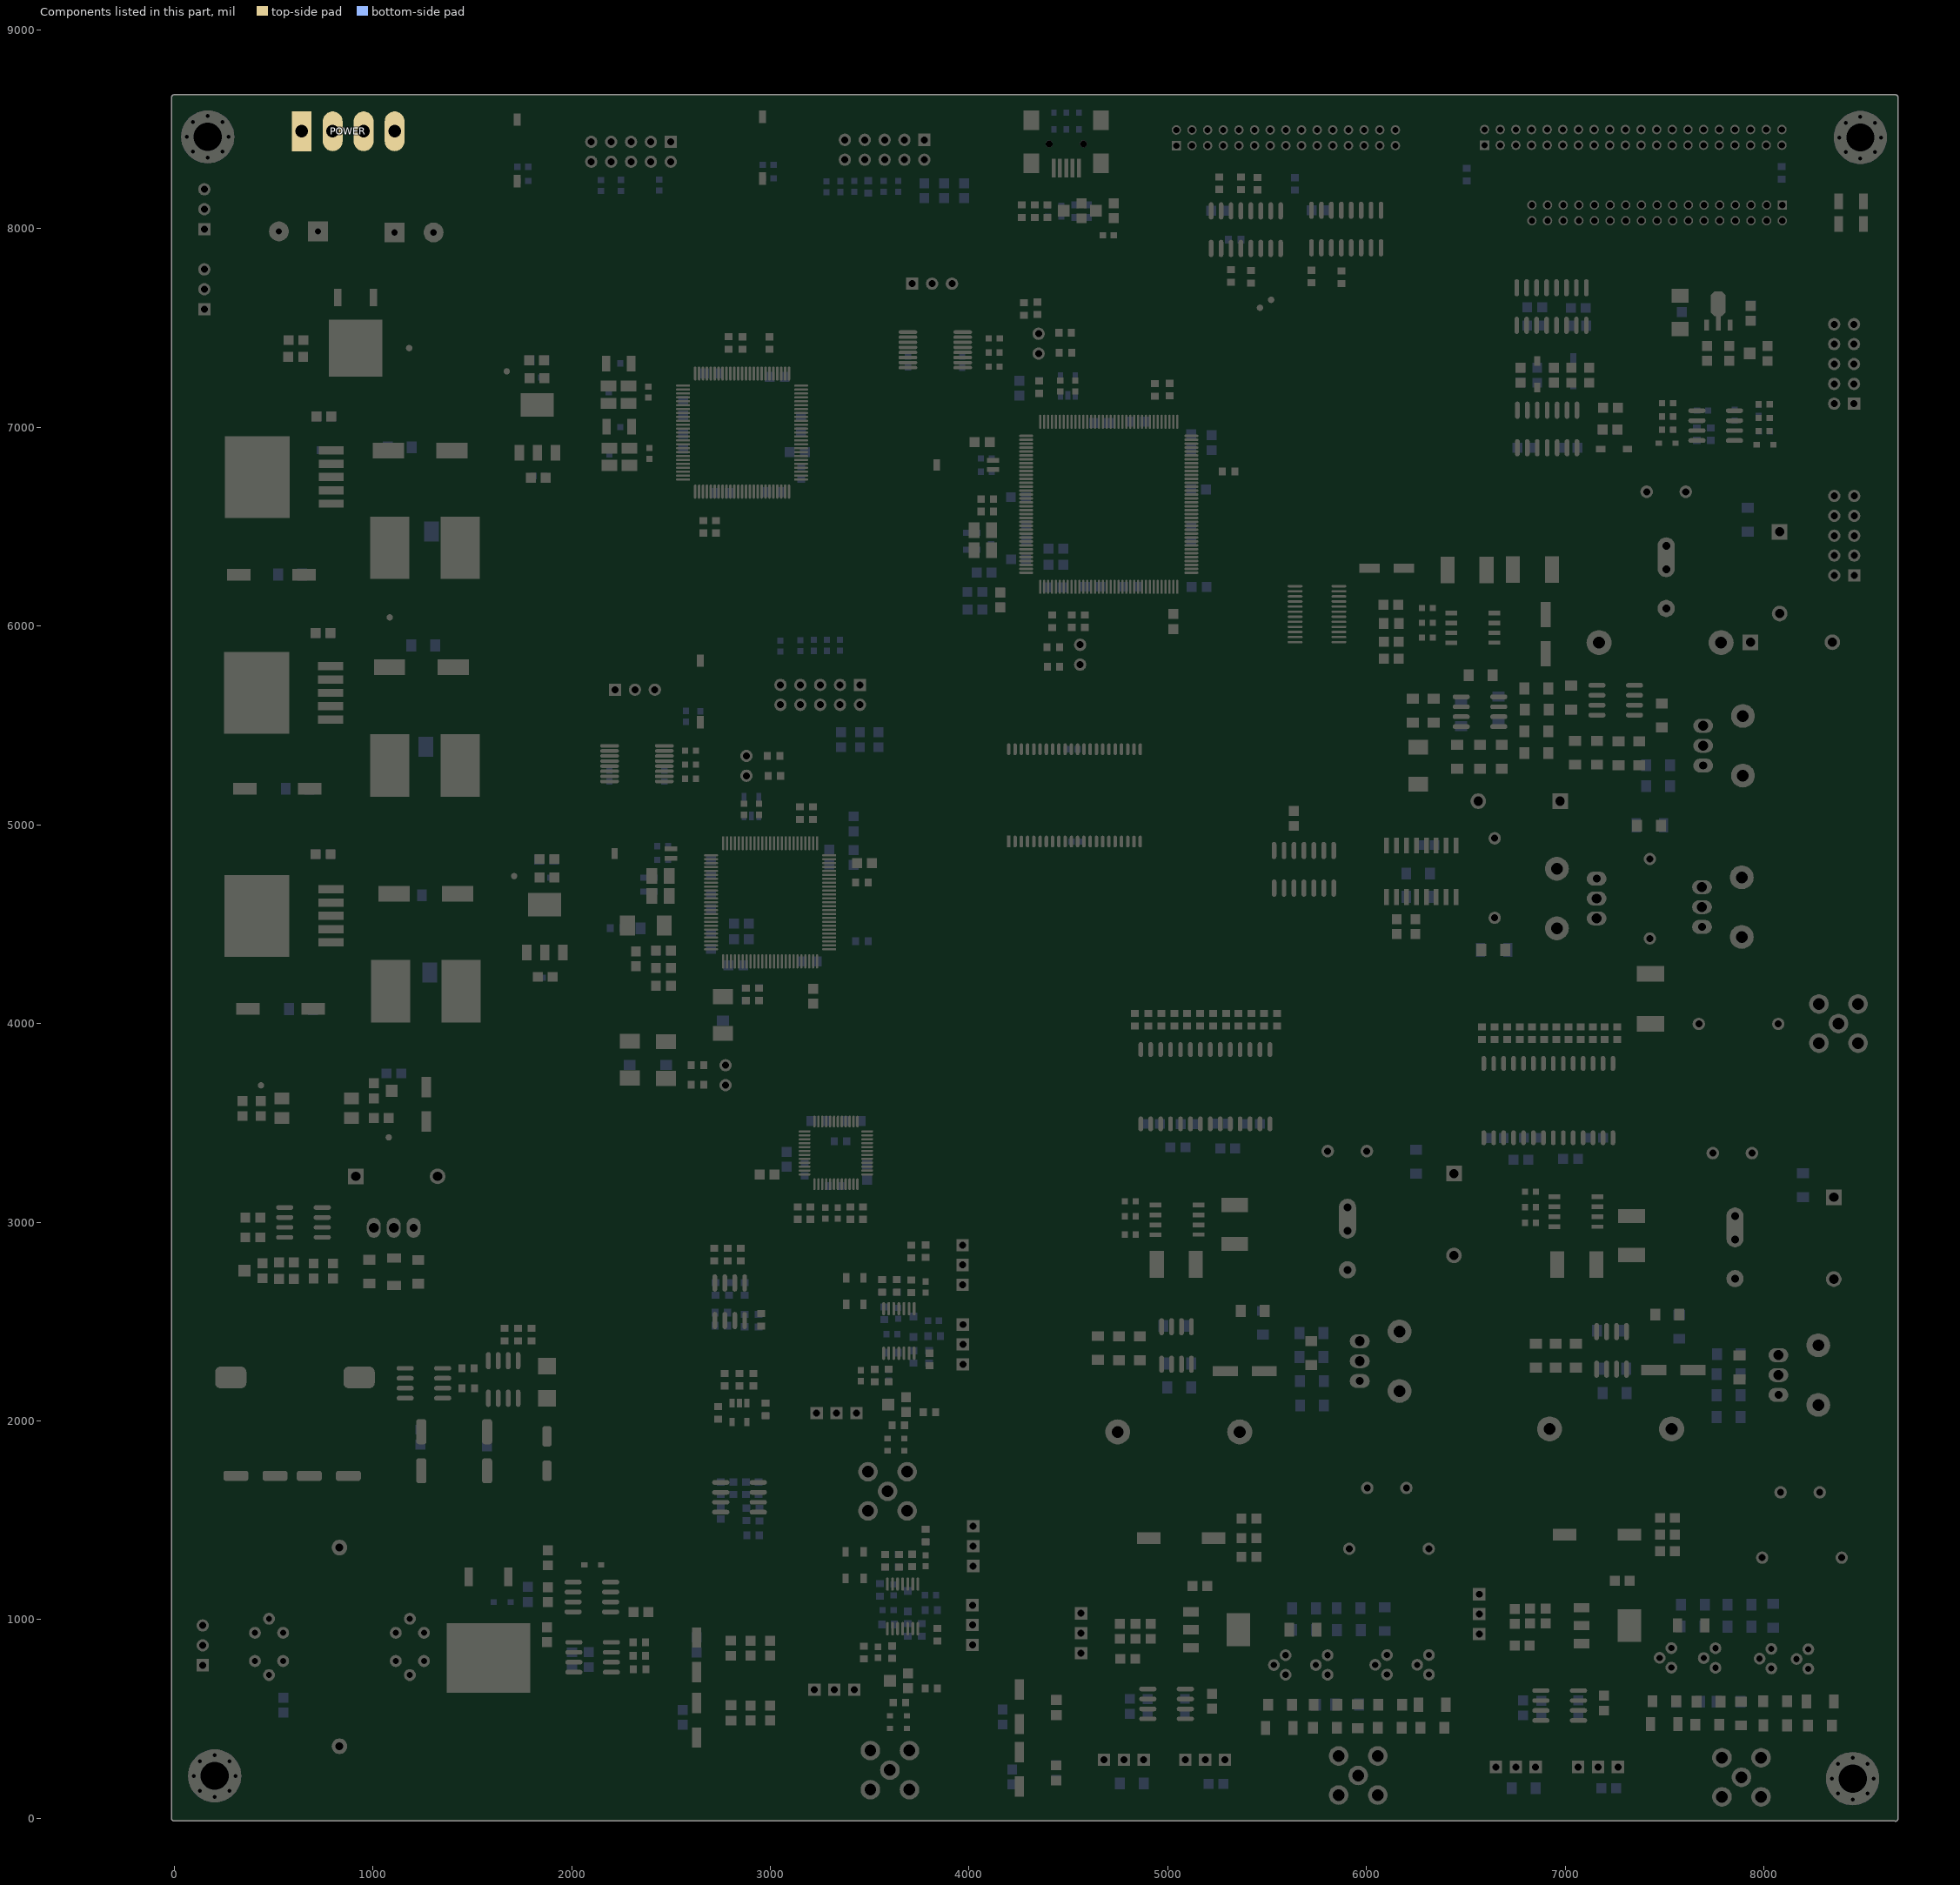
[diagram p0: the components of this part, seen from the top]
# Altium PCB MISC82309.PcbDoc (part 13 of 14)
Units mil, origin at the board's own origin, x right, y up, seen from the top; angles counter-clockwise.
Board outline 8687.03 x 8687.86 mil, 4 copper layers (Top Layer, GND, POWER, Bottom Layer); 747 components, 583 nets, 2530 pads, 1834 vias.

## Polygon pours and split planes (outlines as drawn) (continued)
NetC29_1 on Top Layer "Top Layer-No Net" (solid, remove dead copper, shelved, pour order 1036): 19 vertices, not listed, extent 6047,2224 6178,2381
-12V on Top Layer "TopLayer-No Net" (solid, remove dead copper, shelved, pour order 1050): 39 vertices, not listed, extent 254,4335 1191,4750
+12V on Top Layer "TopLayer-No Net" (solid, remove dead copper, shelved, pour order 1046): 46 vertices, not listed, extent 718,5132 1605,5994
DET-12V on Top Layer "TopLayer-No Net" (solid, remove dead copper, shelved, pour order 1040): 18 vertices, not listed, extent 2898,611 2994,715
DET+12V on Top Layer "TopLayer-No Net" (solid, remove dead copper, shelved, pour order 1035): 18 vertices, not listed, extent 2899,948 2995,1052
NetC78_1 on Top Layer "Top Layer-No Net" (solid, remove dead copper, shelved, pour order 1034): 38 vertices, not listed, extent 698,2782 1044,3278
NetQ22_2 on Top Layer "TopLayer-No Net" (solid, remove dead copper, shelved, pour order 1033): 36 vertices, not listed, extent 1222,605 1798,1002
HV_VCC on Top Layer "TopLayer-No Net" (solid, remove dead copper, shelved, pour order 1039): 64 vertices, not listed, extent 185,894 1324,2286
NetC229_1 on Top Layer "TopLayer-No Net" (solid, remove dead copper, shelved, pour order 1045): 38 vertices, not listed, extent 835,2082 1401,2333
VOCM on Top Layer "Top Layer-No Net" (solid, remove dead copper, shelved, pour order 1032): 4005,2902 4005,2873 4005,2869 4011,2863 4013,2861 4031,2861 4064,2861 4067,2864 4067,2880 4067,2903 4063,2907 4060,2910 4042,2910 4013,2910 4005,2902
VOCM on Top Layer "Top Layer-No Net" (solid, remove dead copper, shelved, pour order 1038): 3866,2916 3866,2898 3866,2885 3870,2881 3877,2874 3896,2874 3913,2874 3916,2877 3916,2891 3916,2917 3911,2922 3910,2923 3899,2923 3873,2923 3866,2916
C_3V3 on Top Layer "Top Layer-No Net" (solid, remove dead copper, shelved, pour order 1044): 39 vertices, not listed, extent 1653,6828 1921,7299
VDD_3V3 on Top Layer "Top Layer-No Net" (solid, remove dead copper, shelved, pour order 1049): 18 vertices, not listed, extent 3785,2987 3842,3081
VDD_3V3 on Top Layer "Top Layer-No Net" (solid, remove dead copper, shelved, pour order 1053): 33 vertices, not listed, extent 1684,4315 1972,4767
VDD_3V3 on Top Layer "Top Layer-No Net" (solid, remove dead copper, shelved, pour order 1056): 22 vertices, not listed, extent 7815,7458 7984,7564
24V_IN on Top Layer "Top Layer-No Net" (solid, remove dead copper, shelved, pour order 1059): 65 vertices, not listed, extent 113,7605 1167,8599
VCC on Top Layer "Top Layer-No Net" (solid, remove dead copper, shelved, pour order 1062): 125 vertices, not listed, extent 716,3452 2015,6937
DC-IN on Top Layer "Top Layer-No Net" (solid, remove dead copper, shelved, pour order 1064): 26 vertices, not listed, extent 1115,1881 1291,2180
DC-IN on Top Layer "Top Layer-No Net" (solid, remove dead copper, shelved, pour order 1065): 34 vertices, not listed, extent 6517,6167 6999,6574
DC-IN on Top Layer "Top Layer-No Net" (solid, remove dead copper, shelved, pour order 1066): 27 vertices, not listed, extent 7319,3404 7623,3676
NetFUSE2_1 on Top Layer "Top Layer-No Net" (solid, remove dead copper, shelved, pour order 1067): 37 vertices, not listed, extent 6304,6220 6460,6578
NetFUSE12_1 on Top Layer "Top Layer-No Net" (solid, remove dead copper, shelved, pour order 1068): 36 vertices, not listed, extent 7101,3125 7408,3487
DC-IN on Top Layer "Top Layer-No Net" (solid, remove dead copper, shelved, pour order 1069): 157 vertices, not listed, extent 76,2961 1120,7550
DC-IN on Top Layer "Top Layer-No Net" (solid, remove dead copper, shelved, pour order 1070): 23 vertices, not listed, extent 238,3549 373,3660
DC-IN on Top Layer "Top Layer-No Net" (solid, remove dead copper, shelved, pour order 1071): 26 vertices, not listed, extent 5206,3405 5505,3629
VCC on Top Layer "Top Layer-No Net" (solid, remove dead copper, shelved, pour order 1072): 30 vertices, not listed, extent 7954,7798 8626,8183
DC-IN on Top Layer "Top Layer-No Net" (solid, remove dead copper, shelved, pour order 1073): 18 vertices, not listed, extent 8405,7923 8558,8076
NetD3_2 on Top Layer "Top Layer-No Net" (solid, remove dead copper, shelved, pour order 1074): 30 vertices, not listed, extent 714,6213 1197,6706
NetD2_2 on Top Layer "Top Layer-No Net" (solid, remove dead copper, shelved, pour order 1075): 26 vertices, not listed, extent 713,5128 1189,5621
NetD4_2 on Top Layer "Top Layer-No Net" (solid, remove dead copper, shelved, pour order 1076): 26 vertices, not listed, extent 714,3987 1196,4498
VDD_3V3 on Top Layer "Top Layer-No Net" (solid, remove dead copper, shelved, pour order 1077): 18 vertices, not listed, extent 2915,3211 2975,3335
NetC411_2 on Top Layer "Top Layer-No Net" (solid, remove dead copper, shelved, pour order 1078): 17 vertices, not listed, extent 2992,3155 3064,3269
-12V on Top Layer "TopLayer-No Net" (solid, remove dead copper, shelved, pour order 1031): 27 vertices, not listed, extent 2574,600 2873,709
-12V on Top Layer "TopLayer-No Net" (solid, remove dead copper, shelved, pour order 1037): 24 vertices, not listed, extent 4121,202 4438,312
-12V on Top Layer "TopLayer-No Net" (solid, remove dead copper, shelved, pour order 1043): 18 vertices, not listed, extent 4607,1308 4681,1408
+12V on Top Layer "TopLayer-No Net" (solid, remove dead copper, shelved, pour order 1048): 66 vertices, not listed, extent 1515,1592 2145,2340
+12V on Top Layer "TopLayer-No Net" (solid, remove dead copper, shelved, pour order 1052): 76 vertices, not listed, extent 2611,390 4437,1140
NetC29_1 on Bottom Layer "Top Layer-No Net" (solid, remove dead copper, shelved, pour order 1047): 19 vertices, not listed, extent 6047,2224 6178,2381
GND on Bottom Layer "Top Layer-No Net" (solid, remove dead copper, shelved, pour order 1042): -572.05,8842.95 -323.05,8593.95 -323.05,-386.05 8993.95,-386.05 9081.95,-298.05 9286.95,-93.05 9286.95,8886.95 -520.05,8886.95 -561.05,8845.95
+12V on Bottom Layer "TopLayer-No Net" (solid, remove dead copper, shelved, pour order 1061): 21 vertices, not listed, extent 1014,5757 1174,5986
-12V on Bottom Layer "TopLayer-No Net" (solid, remove dead copper, shelved, pour order 1058): 23 vertices, not listed, extent 1034,4535 1177,4693
DET-12V on Bottom Layer "TopLayer-No Net" (solid, remove dead copper, shelved, pour order 1055): 19 vertices, not listed, extent 2900,681 2994,720
DET+12V on Bottom Layer "TopLayer-No Net" (solid, remove dead copper, shelved, pour order 1051): 19 vertices, not listed, extent 2901,1014 2995,1053
VOCM on Bottom Layer "Top Layer-No Net" (solid, remove dead copper, shelved, pour order 1079): 26 vertices, not listed, extent 3864,2857 4068,2927
VCC on Bottom Layer "Top Layer-No Net" (solid, remove dead copper, shelved, pour order 1080): 17 vertices, not listed, extent 1887,4202 1984,4265
VCC on Bottom Layer "Top Layer-No Net" (solid, remove dead copper, shelved, pour order 1081): 17 vertices, not listed, extent 1845,6714 1935,6773
VCC on Bottom Layer "Top Layer-No Net" (solid, remove dead copper, shelved, pour order 1082): 21 vertices, not listed, extent 906,6761 1107,6926
NetD3_2 on Bottom Layer "Top Layer-No Net" (solid, remove dead copper, shelved, pour order 1083): 18 vertices, not listed, extent 1042,6413 1159,6651
NetD2_2 on Bottom Layer "Top Layer-No Net" (solid, remove dead copper, shelved, pour order 1084): 18 vertices, not listed, extent 1024,5334 1139,5562
NetD4_2 on Bottom Layer "Top Layer-No Net" (solid, remove dead copper, shelved, pour order 1085): 18 vertices, not listed, extent 1048,4196 1161,4435
-12V on Bottom Layer "TopLayer-No Net" (solid, remove dead copper, shelved, pour order 1054): 141 vertices, not listed, extent 655,204 4260,4693
-12V on Bottom Layer "TopLayer-No Net" (solid, remove dead copper, shelved, pour order 1057): 47 vertices, not listed, extent 4011,216 4682,1411
+12V on Bottom Layer "TopLayer-No Net" (solid, remove dead copper, shelved, pour order 1060): 50 vertices, not listed, extent 6964,7068 8599,8147
+12V on Bottom Layer "TopLayer-No Net" (solid, remove dead copper, shelved, pour order 1063): 6260,323.92 6260,254.41 6270,245.5 6289,228.56 6293,225 6320,225 6393,225 6440,266.88 6440,294.51 6440,347.09 6430,356 6278,356 6265,344.42 6260,339.96 6260,322.14
+18V on Top Layer "TopLayer-No Net" (solid, remove dead copper, pour order 1009): 33 vertices, not listed, extent 7240,2127 7520,2307
NetC266_1 on Top Layer "TopLayer-No Net" (solid, remove dead copper, pour order 1008): 31 vertices, not listed, extent 7897,1593 8605,3388
NetD41_1 on Top Layer "TopLayer-No Net" (solid, remove dead copper, pour order 1007): 32 vertices, not listed, extent 7791,2194 8440,2780
DC-IN on Top Layer "TopLayer-No Net" (solid, remove dead copper, pour order 1006): 22 vertices, not listed, extent 7121,2958 7487,3157
NetFUSE12_2 on Top Layer "TopLayer-No Net" (solid, remove dead copper, pour order 1005): 26 vertices, not listed, extent 7115,2695 7911,3089
+18V on Top Layer "TopLayer-No Net" (solid, remove dead copper, pour order 1004): 28 vertices, not listed, extent 5051,2144 5360,2332
NetC29_1 on Top Layer "TopLayer-No Net" (solid, remove dead copper, pour order 1003): 47 vertices, not listed, extent 5960,1614 6680,3406
NetD5_1 on Top Layer "TopLayer-No Net" (solid, remove dead copper, pour order 1002): 40 vertices, not listed, extent 5826,2238 6499,2890
DC-IN on Top Layer "TopLayer-No Net" (solid, remove dead copper, pour order 1001): 26 vertices, not listed, extent 5118,2919 5537,3164
NetFUSE1_2 on Top Layer "TopLayer-No Net" (solid, remove dead copper, pour order 1000): 26 vertices, not listed, extent 5100,2705 5966,3129
NetD13_1 on Top Layer "Top Layer-No Net" (solid, remove dead copper, pour order 1000): 43 vertices, not listed, extent 7444,5349 8161,6161
NetFUSE2_2 on Top Layer "Top Layer-No Net" (solid, remove dead copper, pour order 1001): 30 vertices, not listed, extent 6554,6201 7594,6531
DC-IN on Top Layer "Top Layer-No Net" (solid, remove dead copper, pour order 1002): 38 vertices, not listed, extent 6606,5900 6997,6385
AMP-12V on Top Layer "Top Layer-No Net" (solid, remove dead copper, pour order 1003): 6134,5843 6134,5802 6139,5797 6142,5794 6169,5794 6241,5794 6249,5802 6249,5819 6249,5859 6241,5867 6208,5867 6138,5867 6134,5863 6134,5843
-12V on Top Layer "Top Layer-No Net" (solid, remove dead copper, pour order 1004): 22 vertices, not listed, extent 6027,6262 6252,6487
+12V on Top Layer "Top Layer-No Net" (solid, remove dead copper, pour order 1005): 49 vertices, not listed, extent 721,5111 1581,5996
+12V on Top Layer "Top Layer-No Net" (solid, remove dead copper, pour order 1006): 62 vertices, not listed, extent 1519,1602 2060,2329
+12V on Top Layer "Top Layer-No Net" (solid, remove dead copper, pour order 1007): 26 vertices, not listed, extent 2401,481 2836,635
+12V on Top Layer "Top Layer-No Net" (solid, remove dead copper, pour order 1008): 26 vertices, not listed, extent 4005,496 4487,717
NetC411_2 on Top Layer "Top Layer-No Net" (solid, remove dead copper, pour order 1009): 17 vertices, not listed, extent 2993,3160 3064,3270
VDD_3V3 on Top Layer "Top Layer-No Net" (solid, remove dead copper, pour order 1010): 17 vertices, not listed, extent 2911,3209 2977,3331
DET+12V on Top Layer "Top Layer-No Net" (solid, remove dead copper, pour order 1011): 18 vertices, not listed, extent 2972,541 3053,661
DET-12V on Top Layer "Top Layer-No Net" (solid, remove dead copper, pour order 1012): 17 vertices, not listed, extent 2967,866.65 3045,979
DET-12V on Top Layer "Top Layer-No Net" (solid, remove dead copper, pour order 1013): 17 vertices, not listed, extent 3274,1164 3334,1227
VDD_3V3 on Top Layer "Top Layer-No Net" (solid, remove dead copper, pour order 1014): 37 vertices, not listed, extent 1674,4315 1966,4771
VCC on Top Layer "Top Layer-No Net" (solid, remove dead copper, pour order 1015): 26 vertices, not listed, extent 1879,4182 2020,4404
C_3V3 on Top Layer "Top Layer-No Net" (solid, remove dead copper, pour order 1016): 42 vertices, not listed, extent 1635,6825 1924,7313
VCC on Top Layer "Top Layer-No Net" (solid, remove dead copper, pour order 1017): 24 vertices, not listed, extent 1843,6706 1980,6915
24V_IN on Top Layer "Top Layer-No Net" (solid, remove dead copper, pour order 1018): 65 vertices, not listed, extent 108,7604 1176,8600
NetC78_1 on Top Layer "Top Layer-No Net" (solid, remove dead copper, pour order 1019): 34 vertices, not listed, extent 697,2781 1044,3286
DC-IN on Top Layer "Top Layer-No Net" (solid, remove dead copper, pour order 1020): 138 vertices, not listed, extent 41,2959 1054,7554
NetD2_2 on Top Layer "Top Layer-No Net" (solid, remove dead copper, pour order 1021): 25 vertices, not listed, extent 710,5114 1194,5619
NetD4_2 on Top Layer "Top Layer-No Net" (solid, remove dead copper, pour order 1022): 25 vertices, not listed, extent 711,3968 1202,4500
-12V on Top Layer "Top Layer-No Net" (solid, remove dead copper, pour order 1023): 42 vertices, not listed, extent 245,4326 1189,4757
NetD3_2 on Top Layer "Top Layer-No Net" (solid, remove dead copper, pour order 1024): 25 vertices, not listed, extent 715,6198 1205,6707
VCC on Top Layer "Top Layer-No Net" (solid, remove dead copper, pour order 1025): 41 vertices, not listed, extent 716,6191 1584,6937
VCC on Top Layer "Top Layer-No Net" (solid, remove dead copper, pour order 1026): 22 vertices, not listed, extent 1052,3444 1397,3568
DC-IN on Top Layer "Top Layer-No Net" (solid, remove dead copper, pour order 1027): 25 vertices, not listed, extent 8439,7889 8534,8067
DC-IN on Top Layer "Top Layer-No Net" (solid, remove dead copper, pour order 1028): 24 vertices, not listed, extent 1104,1879 1279,2179
VCC on Top Layer "Top Layer-No Net" (solid, remove dead copper, pour order 1029): 42 vertices, not listed, extent 7915,7777 8615,8184
VDD_3V3 on Top Layer "Top Layer-No Net" (solid, remove dead copper, pour order 1030): 4697,3692 4697,3642 4706,3633 4713,3626 4725,3626 4751,3626 4757,3632 4767,3642 4767,3648 4767,3672 4754,3685 4741,3698 4735,3698 4703,3698 4697,3692
VDD_3V3 on Top Layer "Top Layer-No Net" (solid, remove dead copper, pour order 1031): 18 vertices, not listed, extent 4742,3769 4786,3827
VCC on Top Layer "Top Layer-No Net" (solid, remove dead copper, pour order 1032): 18 vertices, not listed, extent 2740,2219 2802,2298
-12V on Top Layer "Top Layer-No Net" (solid, remove dead copper, pour order 1033): 22 vertices, not listed, extent 4095,100 4477,221
-12V on Top Layer "Top Layer-No Net" (solid, remove dead copper, pour order 1034): 21 vertices, not listed, extent 2600,855 2836,986
NetQ22_2 on Top Layer "Top Layer-No Net" (solid, remove dead copper, pour order 1035): 29 vertices, not listed, extent 1221,613 1806,992
NetC229_1 on Top Layer "Top Layer-No Net" (solid, remove dead copper, pour order 1036): 42 vertices, not listed, extent 845,2090 1402,2288
HV_VCC on Top Layer "Top Layer-No Net" (solid, remove dead copper, pour order 1037): 54 vertices, not listed, extent 174,896 1334,2292
GND on Top Layer "Top Layer-No Net" (solid, remove dead copper, pour order 1038): 40 vertices, not listed, extent 3403,66 3816,926
GND on Top Layer "Top Layer-No Net" (solid, remove dead copper, pour order 1039): 38 vertices, not listed, extent 3398,1474 3778,2311
GND on Top Layer "Top Layer-No Net" (solid, remove dead copper, pour order 1041): 39 vertices, not listed, extent 244,6534 996,6991
GND on Top Layer "Top Layer-No Net" (solid, remove dead copper, pour order 1042): 34 vertices, not listed, extent 1218,6666 1823,7254
GND on Top Layer "Top Layer-No Net" (solid, remove dead copper, pour order 1043): 18 vertices, not listed, extent 245,6202 477,6410
GND on Top Layer "Top Layer-No Net" (solid, remove dead copper, pour order 1044): 18 vertices, not listed, extent 924,2581 1285,2722
GND on Top Layer "Top Layer-No Net" (solid, remove dead copper, pour order 1045): 18 vertices, not listed, extent 1175,1614 1622,1816
GND on Top Layer "Top Layer-No Net" (solid, remove dead copper, pour order 1046): 18 vertices, not listed, extent 143,1661 381,1784
GND on Top Layer "Top Layer-No Net" (solid, remove dead copper, pour order 1047): 18 vertices, not listed, extent 806,1663 1021,1775
GND on Top Layer "Top Layer-No Net" (solid, remove dead copper, pour order 1048): 38 vertices, not listed, extent 240,5448 1086,5889
GND on Top Layer "Top Layer-No Net" (solid, remove dead copper, pour order 1049): 18 vertices, not listed, extent 253,5118 449,5310
GND on Top Layer "Top Layer-No Net" (solid, remove dead copper, pour order 1050): 20 vertices, not listed, extent 1276,5669 1685,6098
GND on Top Layer "Top Layer-No Net" (solid, remove dead copper, pour order 1051): 25 vertices, not listed, extent 708,4584 988,4752
GND on Top Layer "Top Layer-No Net" (solid, remove dead copper, pour order 1052): 39 vertices, not listed, extent 1331,3968 1858,4709
GND on Top Layer "Top Layer-No Net" (solid, remove dead copper, pour order 1053): 266,4231 266,4060 288,4038 298,4028 328,4028 436,4028 440,4032 446,4038 446,4064 446,4225 426,4245 421,4250 390,4250 285,4250 266,4231
GND on Top Layer "Top Layer-No Net" (solid, remove dead copper, pour order 1054): 17 vertices, not listed, extent 1411,1159 1552,1354
GND on Top Layer "Top Layer-No Net" (solid, remove dead copper, pour order 1055): 18 vertices, not listed, extent 2568,678 2733,794
GND on Top Layer "Top Layer-No Net" (solid, remove dead copper, pour order 1056): 2553,444 2553,359 2561,351 2568,344 2620,344 2728,344 2736,352 2738,354 2738,384 2738,459 2731,466 2727,470 2640,470 2578,470 2553,445
GND on Top Layer "Top Layer-No Net" (solid, remove dead copper, pour order 1057): 19 vertices, not listed, extent 4164,279 4351,536
GND on Top Layer "Top Layer-No Net" (solid, remove dead copper, pour order 1058): 18 vertices, not listed, extent 4756,1345 4983,1552
GND on Top Layer "Top Layer-No Net" (solid, remove dead copper, pour order 1059): 18 vertices, not listed, extent 6910,1351 7107,1577
GND on Top Layer "Top Layer-No Net" (solid, remove dead copper, pour order 1060): 5418,2286 5418,2188 5429,2177 5445,2161 5514,2161 5611,2161 5619,2169 5631,2181 5631,2208 5631,2266 5609,2288 5591,2306 5550,2306 5439,2306 5419,2286
GND on Top Layer "Top Layer-No Net" (solid, remove dead copper, pour order 1061): 18 vertices, not listed, extent 7577,2137 7718,2310
GND on Top Layer "Top Layer-No Net" (solid, remove dead copper, pour order 1062): 18 vertices, not listed, extent 6162,5076 6343,5252
GND on Top Layer "Top Layer-No Net" (solid, remove dead copper, pour order 1063): 18 vertices, not listed, extent 6836,5987 7047,6129
GND on Top Layer "Top Layer-No Net" (solid, remove dead copper, pour order 1064): 30 vertices, not listed, extent 5906,6074 6112,6386
GND on Top Layer "Top Layer-No Net" (solid, remove dead copper, pour order 1065): 18 vertices, not listed, extent 7438,7445 7635,7540
VDD_3V3 on Top Layer "Top Layer-No Net" (solid, remove dead copper, pour order 1066): 19 vertices, not listed, extent 7812,7464 7985,7564
GND on Top Layer "Top Layer-No Net" (solid, remove dead copper, pour order 1067): 17 vertices, not listed, extent 7904,7585 8045,7652
GND on Top Layer "Top Layer-No Net" (solid, remove dead copper, pour order 1068): 19 vertices, not listed, extent 1834,7199 1927,7278
GND on Top Layer "Top Layer-No Net" (solid, remove dead copper, pour order 1069): 18 vertices, not listed, extent 1885,4682 1979,4770
GND on Top Layer "Top Layer-No Net" (solid, remove dead copper, pour order 1070): 22 vertices, not listed, extent 1151,435 1260,754
NetC54_1 on Bottom Layer "Top Layer-No Net" (solid, remove dead copper, pour order 1073): 45 vertices, not listed, extent 7566,5866 8132,6710
AMP-12V on Bottom Layer "Top Layer-No Net" (solid, remove dead copper, pour order 1074): 6200,5851 6200,5807 6207,5800 6213,5794 6238,5794 6239,5794 6249,5804 6251,5806 6251,5831 6251,5856 6240,5867 6216,5867 6207,5867 6200,5860 6200,5851
-12V on Bottom Layer "Top Layer-No Net" (solid, remove dead copper, pour order 1075): 6028,6476 6028,6439 6032,6435 6064,6403 6075,6403 6087,6403 6093,6409 6094,6410 6094,6430 6094,6477 6089,6482 6086,6485 6073,6485 6037,6485 6028,6476
+12V on Bottom Layer "Top Layer-No Net" (solid, remove dead copper, pour order 1076): 18 vertices, not listed, extent 6259,236 6488,397
DET+12V on Bottom Layer "Top Layer-No Net" (solid, remove dead copper, pour order 1077): 18 vertices, not listed, extent 2977,603 3049,666
DET-12V on Bottom Layer "Top Layer-No Net" (solid, remove dead copper, pour order 1078): 2975,973 2975,930 2980,925 2983,922 2996,922 3035,922 3038,925 3044,931 3044,941 3044,970 3033,981 3029,985 3019,985 2987,985 2975,973
DET-12V on Bottom Layer "Top Layer-No Net" (solid, remove dead copper, pour order 1079): 17 vertices, not listed, extent 3271,1166 3342,1235
NetD2_2 on Bottom Layer "Top Layer-No Net" (solid, remove dead copper, pour order 1080): 18 vertices, not listed, extent 1021,5327 1139,5564
NetD4_2 on Bottom Layer "Top Layer-No Net" (solid, remove dead copper, pour order 1081): 18 vertices, not listed, extent 1041,4192 1167,4427
-12V on Bottom Layer "Top Layer-No Net" (solid, remove dead copper, pour order 1082): 30 vertices, not listed, extent 1036,4190 1354,4688
NetD3_2 on Bottom Layer "Top Layer-No Net" (solid, remove dead copper, pour order 1083): 18 vertices, not listed, extent 1043,6414 1159,6651
-12V on Bottom Layer "Top Layer-No Net" (solid, remove dead copper, pour order 1084): 18 vertices, not listed, extent 4093.5,146.5 4190.5,212.5
-12V on Bottom Layer "Top Layer-No Net" (solid, remove dead copper, pour order 1085): 18 vertices, not listed, extent 2654,919 2754,983
GND on Bottom Layer "Top Layer-No Net" (solid, remove dead copper, pour order 1086): 36 vertices, not listed, extent 1212,6395 1716,7252
GND on Bottom Layer "Top Layer-No Net" (solid, remove dead copper, pour order 1087): 31 vertices, not listed, extent 1224,5332 1673,6100
GND on Bottom Layer "Top Layer-No Net" (solid, remove dead copper, pour order 1088): 19 vertices, not listed, extent 485,417 599,560
GND on Bottom Layer "Top Layer-No Net" (solid, remove dead copper, pour order 1089): 23 vertices, not listed, extent 5565,2007 5699,2304
GND on Bottom Layer "Top Layer-No Net" (solid, remove dead copper, pour order 1090): 30 vertices, not listed, extent 7655,1976 7801,2228
GND on Bottom Layer "Top Layer-No Net" (solid, remove dead copper, pour order 1091): 18 vertices, not listed, extent 7439,7457 7642,7608
GND on Bottom Layer "Top Layer-No Net" (solid, remove dead copper, pour order 1092): 7861,6669 7861,6587 7878,6570 7883,6565 7920,6565 7972,6565 7980,6573 7984,6577 7984,6651 7984,6673 7972,6685 7967,6690 7918,6690 7880,6690 7861,6671
GND on Bottom Layer "Top Layer-No Net" (solid, remove dead copper, pour order 1093): 7907,7638 7907,7591 7911,7587 7912,7586 7917,7586 8033,7586 8038,7591 8044,7597 8044,7617 8044,7646 8041,7649 8037,7653 8024,7653 7922,7653 7907,7638
GND on Bottom Layer "Top Layer-No Net" (solid, remove dead copper, pour order 1094): -342,8771 -342,-164 -127,-379 9581,-379 9581,8479 9315,8745 9277,8783 -329,8783
VDD_3V3 on POWER (split plane): 306 vertices, not listed, extent 1676.56,909.56 8280.44,8550.44
DC-IN on POWER (split plane): 222 vertices, not listed, extent 7.58,7.58 8654.42,8295.68
VCC on POWER (split plane): 313 vertices, not listed, extent 888.56,1153.56 8047.44,8550.44
+18V on POWER (split plane): 149 vertices, not listed, extent 1018.56,387.56 8053.44,5814.44
C_3V3 on POWER (split plane): 87 vertices, not listed, extent 7.58,6190.56 8654.42,8653.84
+12V on POWER (split plane): 115 vertices, not listed, extent 7.58,247.56 6474,6566.71
NetC411_2 on POWER (split plane): 43 vertices, not listed, extent 2964.56,3017.56 3677.44,3489.44
GND on GND (split plane): 8654.42,7.58 7.58,7.58 7.58,8653.84 8654.42,8653.84

## Keep-outs
Keep-Out Layer:
  lines w25: 8661.42,0 0,0 0,8661.42 8661.42,8661.42 ; 8662,-1.42 8662,8660

## Other copper
Bottom Layer:
  pour cut-out: -77,375 -75,375 70,520 1236,520 1312,596 1312,1495 1395,1578 1959,1578 2036,1655 2036,2531 1997,2570 1798,2570 1690,2678 1690,7072 1498,7264 1498,8541 1687,8730 1531,8886 79,8886 -515,8292 -515,813
  pour cut-out: -78,394 -67,383 70,520 1236,520 1312,596 1312,1145 1214,1243 60,1243 -3,1306 -51,1306 -78,1279
  pour cut-out: 7327,3871 7405,3793 8503,3793 8555,3741 8571,3741 8571,4251 8567,4255 8466,4154 7591,4154 7554,4191 7554,4305 7537,4322 7535,4320 7351,4320 7327,4296
  pour cut-out: 4601,1217 4557,1173 4428,1173 4402,1147 4402,780 4341,719 4091,719 4003,631 4003,78 3913,-12 3974,-73 4039,-73 4043,-77 8706,-77 8796,13 8796,3545 8700,3641 8612,3553 7649,3553 7566,3470 7566,3256 7513,3203 6603,3203 6483,3323 6483,3553 6452,3584 5703,3584 5668,3549 5668,3278 5581,3191 4629,3191 4601,3163
GND (plane layer: these items are gaps in the copper):
  region: 8,466 63,521 1235,521 1312,598 1312,1146 1216,1242 59,1242 9,1292 8,1291